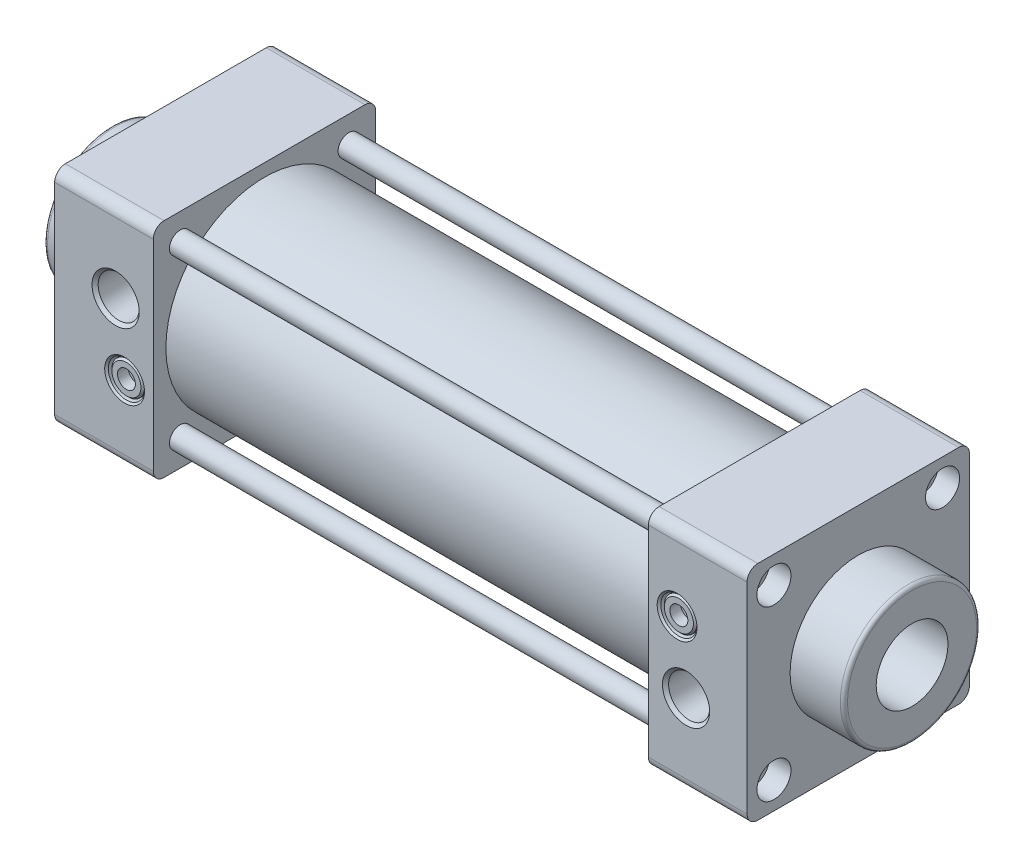
from build123d import *

# Parameters (mm, degrees)
BOSS_EXTRUDE1_DEPTH  = 27.5
SKETCH2_R            = 27.5
BOSS_EXTRUDE2_DEPTH  = 138
BOSS_EXTRUDE3_START  = -27.5
BOSS_EXTRUDE3_DEPTH  = 27.5
LPATTERN1_COUNT      = 2
LPATTERN1_PITCH      = 47
LPATTERN1_COUNT_DIR2 = 2
LPATTERN1_PITCH_DIR2 = 47
LPATTERN2_COUNT      = 2
LPATTERN2_PITCH      = 47
LPATTERN2_COUNT_DIR2 = 2
LPATTERN2_PITCH_DIR2 = 47
SKETCH8_W            = 138
SKETCH8_H            = 3
LPATTERN3_COUNT      = 2
LPATTERN3_PITCH      = 47
LPATTERN3_COUNT_DIR2 = 2
LPATTERN3_PITCH_DIR2 = 47


with BuildPart() as part:
    # Sketch1 → Boss-Extrude1 (new body)
    with BuildSketch(Plane(origin=(0, 0, 0), x_dir=(0, 0, -1), z_dir=(1, 0, 0))):
        with BuildLine():
            Line((-28, -31), (28, -31))
            ThreePointArc((28, -31), (30.121320344, -30.121320344), (31, -28))
            Line((31, -28), (31, 28))
            ThreePointArc((31, 28), (30.121320344, 30.121320344), (28, 31))
            Line((28, 31), (-28, 31))
            ThreePointArc((-28, 31), (-30.121320344, 30.121320344), (-31, 28))
            Line((-31, 28), (-31, -28))
            ThreePointArc((-31, -28), (-30.121320344, -30.121320344), (-28, -31))
        make_face()
    extrude(amount=BOSS_EXTRUDE1_DEPTH)

    # Sketch2 → Boss-Extrude2 (add)
    with BuildSketch(Plane(origin=(27.5, 0, 0), x_dir=(0, 0, -1), z_dir=(1, 0, 0))):
        Circle(SKETCH2_R)
    extrude(amount=BOSS_EXTRUDE2_DEPTH)

    # Sketch3 → Boss-Extrude3 (add)
    with BuildSketch(Plane(origin=(193, 0, 0), x_dir=(0, 0, -1), z_dir=(1, 0, 0)).offset(BOSS_EXTRUDE3_START)):
        with BuildLine():
            Line((-28, -31), (28, -31))
            ThreePointArc((28, -31), (30.121320344, -30.121320344), (31, -28))
            Line((31, -28), (31, 28))
            ThreePointArc((31, 28), (30.121320344, 30.121320344), (28, 31))
            Line((28, 31), (-28, 31))
            ThreePointArc((-28, 31), (-30.121320344, 30.121320344), (-31, 28))
            Line((-31, 28), (-31, -28))
            ThreePointArc((-31, -28), (-30.121320344, -30.121320344), (-28, -31))
        make_face()
    extrude(amount=BOSS_EXTRUDE3_DEPTH)

    # Sketch4 → Cut-Revolve1 (revolve, cut)
    with BuildSketch(Plane.XY.offset(23.5), mode=Mode.PRIVATE) as cut_revolve1_sk:
        Polygon((17, -23.5), (17, -25.9585), (6.5415, -25.9585), (6, -26.5), (6, -28.25), (0, -28.25), (0, -23.5), align=None)
    cut_revolve1 = revolve(cut_revolve1_sk.sketch.rotate(Axis((0, -23.5, 23.5), (1, 0, 0)), 270), axis=Axis((0, -23.5, 23.5), (1, 0, 0)), mode=Mode.SUBTRACT)

    # LPattern1: Cut-Revolve1 2 × 2
    with Locations(*[(0, j * LPATTERN1_PITCH_DIR2, -i * LPATTERN1_PITCH) for i in range(LPATTERN1_COUNT) for j in range(LPATTERN1_COUNT_DIR2) if (i, j) != (0, 0)]):
        add(cut_revolve1, mode=Mode.SUBTRACT)

    # Sketch6 → Cut-Revolve2 (revolve, cut)
    with BuildSketch(Plane.XY.offset(23.5), mode=Mode.PRIVATE) as cut_revolve2_sk:
        Polygon((193, -23.5), (193, -28.25), (187, -28.25), (187, -26.5), (186.4585, -25.9585), (176, -25.9585), (176, -23.5), align=None)
    cut_revolve2 = revolve(cut_revolve2_sk.sketch.rotate(Axis((176, -23.5, 23.5), (1, 0, 0)), 270), axis=Axis((176, -23.5, 23.5), (1, 0, 0)), mode=Mode.SUBTRACT)

    # LPattern2: Cut-Revolve2 2 × 2
    with Locations(*[(0, j * LPATTERN2_PITCH_DIR2, -i * LPATTERN2_PITCH) for i in range(LPATTERN2_COUNT) for j in range(LPATTERN2_COUNT_DIR2) if (i, j) != (0, 0)]):
        add(cut_revolve2, mode=Mode.SUBTRACT)

    # Sketch8 → Revolve1 (revolve)
    with BuildSketch(Plane.XY.offset(23.5), mode=Mode.PRIVATE) as revolve1_sk:
        with Locations((96.5, -22)):
            Rectangle(SKETCH8_W, SKETCH8_H)
    revolve1 = revolve(revolve1_sk.sketch.rotate(Axis((165.5, -23.5, 23.5), (-1, 0, 0)), 270), axis=Axis((165.5, -23.5, 23.5), (-1, 0, 0)))

    # LPattern3: Revolve1 2 × 2
    with Locations(*[(0, j * LPATTERN3_PITCH_DIR2, -i * LPATTERN3_PITCH) for i in range(LPATTERN3_COUNT) for j in range(LPATTERN3_COUNT_DIR2) if (i, j) != (0, 0)]):
        add(revolve1)

    # Sketch10 → Revolve2 (revolve)
    with BuildSketch(Plane.XY, mode=Mode.PRIVATE) as revolve2_sk:
        with BuildLine():
            Line((165.5, 0), (165.5, 19))
            Line((165.5, 19), (207, 19))
            ThreePointArc((207, 19), (207.707106781, 18.707106781), (208, 18))
            Line((208, 18), (208, 0))
            Line((208, 0), (165.5, 0))
        make_face()
    revolve(revolve2_sk.sketch.rotate(Axis((208, 0, 0), (-1, 0, 0)), 270), axis=Axis((208, 0, 0), (-1, 0, 0)))

    # Sketch11 → Cut-Revolve3 (revolve, cut)
    with BuildSketch(Plane(origin=(17, 0, 0), x_dir=(0, 0, -1), z_dir=(1, 0, 0)), mode=Mode.PRIVATE) as cut_revolve3_sk:
        Polygon((-31, 8.5), (-31, 15.0785), (-30.144, 14.2225), (-15.2116, 14.2225), (-15.2116, 8.5), align=None)
    revolve(cut_revolve3_sk.sketch.rotate(Axis((17, 8.5, 15.2116), (0, 0, 1)), 270), axis=Axis((17, 8.5, 15.2116), (0, 0, 1)), mode=Mode.SUBTRACT)

    # Sketch12 → Cut-Revolve4 (revolve, cut)
    with BuildSketch(Plane(origin=(176, 0, 0), x_dir=(0, 0, -1), z_dir=(1, 0, 0)), mode=Mode.PRIVATE) as cut_revolve4_sk:
        Polygon((-31, -8.5), (-31, -1.9215), (-30.144, -2.7775), (-15.2116, -2.7775), (-15.2116, -8.5), align=None)
    revolve(cut_revolve4_sk.sketch.rotate(Axis((176, -8.5, 15.2116), (0, 0, 1)), 270), axis=Axis((176, -8.5, 15.2116), (0, 0, 1)), mode=Mode.SUBTRACT)

    # Sketch13 → Cut-Revolve5 (revolve, cut)
    with BuildSketch(Plane(origin=(19.5, 0, 0), x_dir=(0, 0, -1), z_dir=(1, 0, 0)), mode=Mode.PRIVATE) as cut_revolve5_sk:
        Polygon((-31, -10), (-31, -4.45), (-30.5, -4.95), (-27.5, -4.95), (-27.5, -5.45), (-30, -5.45), (-30.5, -5.95), (-30.5, -7.5), (-27.5, -7.5), (-27.5, -10), align=None)
    revolve(cut_revolve5_sk.sketch.rotate(Axis((19.5, -10, 27.5), (0, 0, 1)), 270), axis=Axis((19.5, -10, 27.5), (0, 0, 1)), mode=Mode.SUBTRACT)

    # Sketch14 → Cut-Revolve6 (revolve, cut)
    with BuildSketch(Plane(origin=(173.5, 0, 0), x_dir=(0, 0, -1), z_dir=(1, 0, 0)), mode=Mode.PRIVATE) as cut_revolve6_sk:
        Polygon((-31, 10), (-31, 15.55), (-30.5, 15.05), (-27.5, 15.05), (-27.5, 14.55), (-30, 14.55), (-30.5, 14.05), (-30.5, 12.5), (-27.5, 12.5), (-27.5, 10), align=None)
    revolve(cut_revolve6_sk.sketch.rotate(Axis((173.5, 10, 27.5), (0, 0, 1)), 270), axis=Axis((173.5, 10, 27.5), (0, 0, 1)), mode=Mode.SUBTRACT)

    # Sketch15 → Revolve3 (revolve)
    with BuildSketch(Plane.XY, mode=Mode.PRIVATE) as revolve3_sk:
        with BuildLine():
            Line((-15, 0), (-15, 18))
            ThreePointArc((-15, 18), (-14.707106781, 18.707106781), (-14, 19))
            Line((-14, 19), (0, 19))
            Line((0, 19), (0, 0))
            Line((0, 0), (-15, 0))
        make_face()
    revolve(revolve3_sk.sketch.rotate(Axis((0, 0, 0), (-1, 0, 0)), 270), axis=Axis((0, 0, 0), (-1, 0, 0)))

    # Sketch16 → Cut-Revolve7 (revolve, cut)
    with BuildSketch(Plane.XY, mode=Mode.PRIVATE) as cut_revolve7_sk:
        Polygon((-20, 0), (-20, 10), (3, 10), (3, 14.2), (33, 14.2), (33, 25), (160, 25), (160, 14.2), (190, 14.2), (190, 10), (213, 10), (213, 0), align=None)
    revolve(cut_revolve7_sk.sketch.rotate(Axis((213, 0, 0), (-1, 0, 0)), 270), axis=Axis((213, 0, 0), (-1, 0, 0)), mode=Mode.SUBTRACT)


solid = part.part
